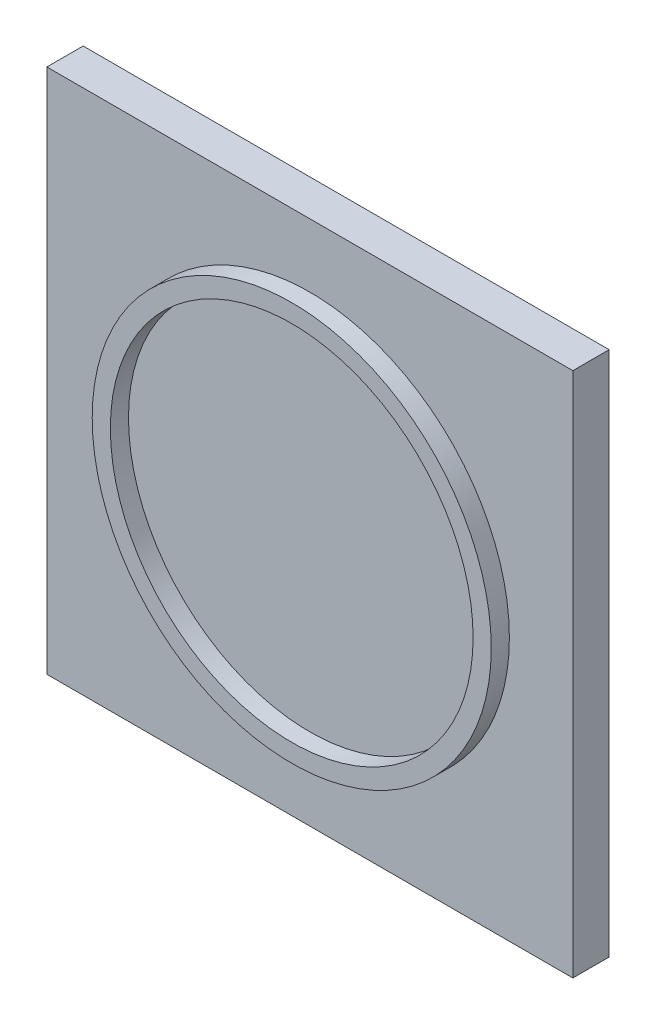
from build123d import *

# Parameters (mm, degrees)
SKETCH1_W           = 145
SKETCH1_H           = 145
BOSS_EXTRUDE1_DEPTH = 10
SKETCH2_R           = 55
SKETCH2_R_2         = 50
BOSS_EXTRUDE2_DEPTH = 5


with BuildPart() as part:
    # Sketch1 → Boss-Extrude1 (new body)
    with BuildSketch(Plane.XY):
        with Locations((72.5, 72.5)):
            Rectangle(SKETCH1_W, SKETCH1_H)
    extrude(amount=BOSS_EXTRUDE1_DEPTH)

    # Sketch2 → Boss-Extrude2 (add)
    with BuildSketch(Plane.XY.offset(10)):
        with Locations(Location((72.5, 72.5, 0), (0, 0, 180))):
            Circle(SKETCH2_R)
        with Locations((72.5, 72.5)):
            Circle(SKETCH2_R_2, mode=Mode.SUBTRACT)
    extrude(amount=BOSS_EXTRUDE2_DEPTH)


solid = part.part
